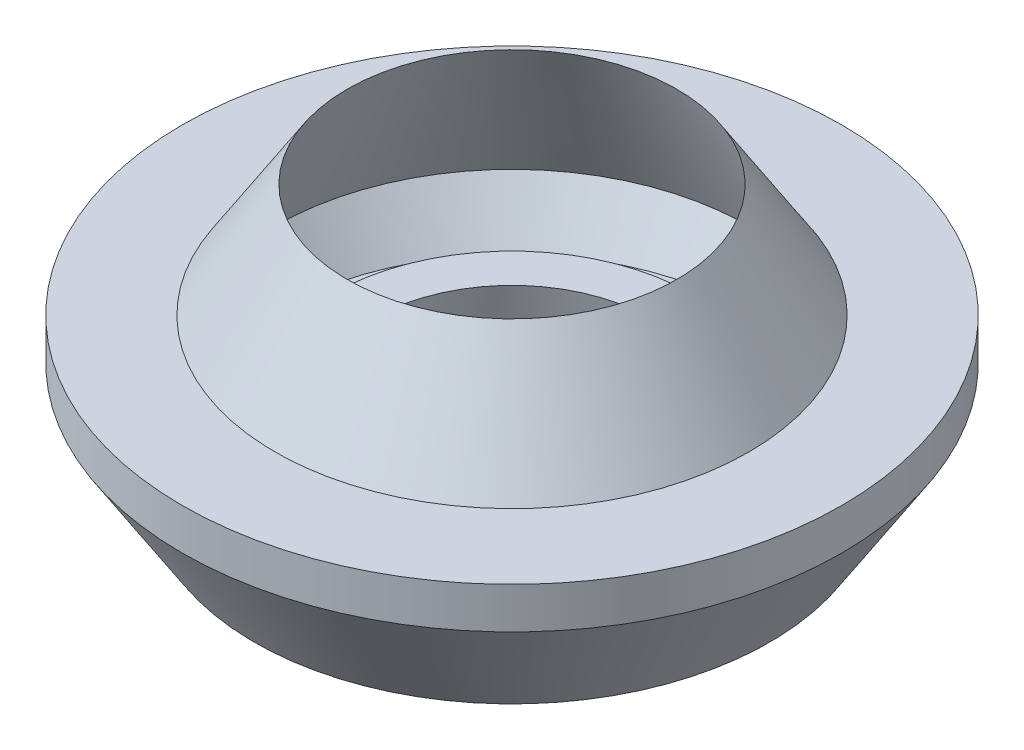
SolidWorks part; units mm, degrees
material "橡胶"
ref_plane "Front Plane" through (0, 0, 0) normal (0, 0, 1) x (1, 0, 0)
ref_plane "Top Plane" through (0, 0, 0) normal (0, 1, 0) x (1, 0, 0)
ref_plane "Right Plane" through (0, 0, 0) normal (1, 0, 0) x (0, 0, -1)
sketch "Sketch1" plane through (0, 0, 0) normal (0, 0, 1) x (1, 0, 0)
  line L0 (0, 12.9153) -> (0, -11.3198) construction
  line L1 (-18.6998, 0) -> (8.8958, 0) construction
  line L2 (16, 26) -> (23, 15)
  line L3 (23, 15) -> (32, 15)
  line L4 (32, 15) -> (32, 11)
  line L5 (32, 11) -> (25, 0)
  line L6 (25, 0) -> (15, 0)
  line L7 (15, 0) -> (13.45, 8)
  line L8 (13.45, 8) -> (17.5244, 8)
  line L9 (17.5244, 8) -> (18.2994, 4)
  line L10 (18.2994, 4) -> (22.8042, 4)
  line L11 (22.8042, 4) -> (27.2588, 11)
  line L12 (27.2588, 11) -> (22.9946, 11)
  line L13 (22.9946, 11) -> (16, 26)
  dimension "D1" = 4
  dimension "D2" = 4
  dimension "D3" = 4
  dimension "D4" = 4
  dimension "D5" = 25
  dimension "D6" = 15
  dimension "D7" = 26
  dimension "D8" = 64
  dimension "D9" = 46
  dimension "D10" = 32
  dimension "D11" = 50
  dimension "D12" = 30
  dimension "D13" = 26.9
  dimension "D14" = 8
revolve "Revolve1" add sketch "Sketch1" angle 360 about L0
